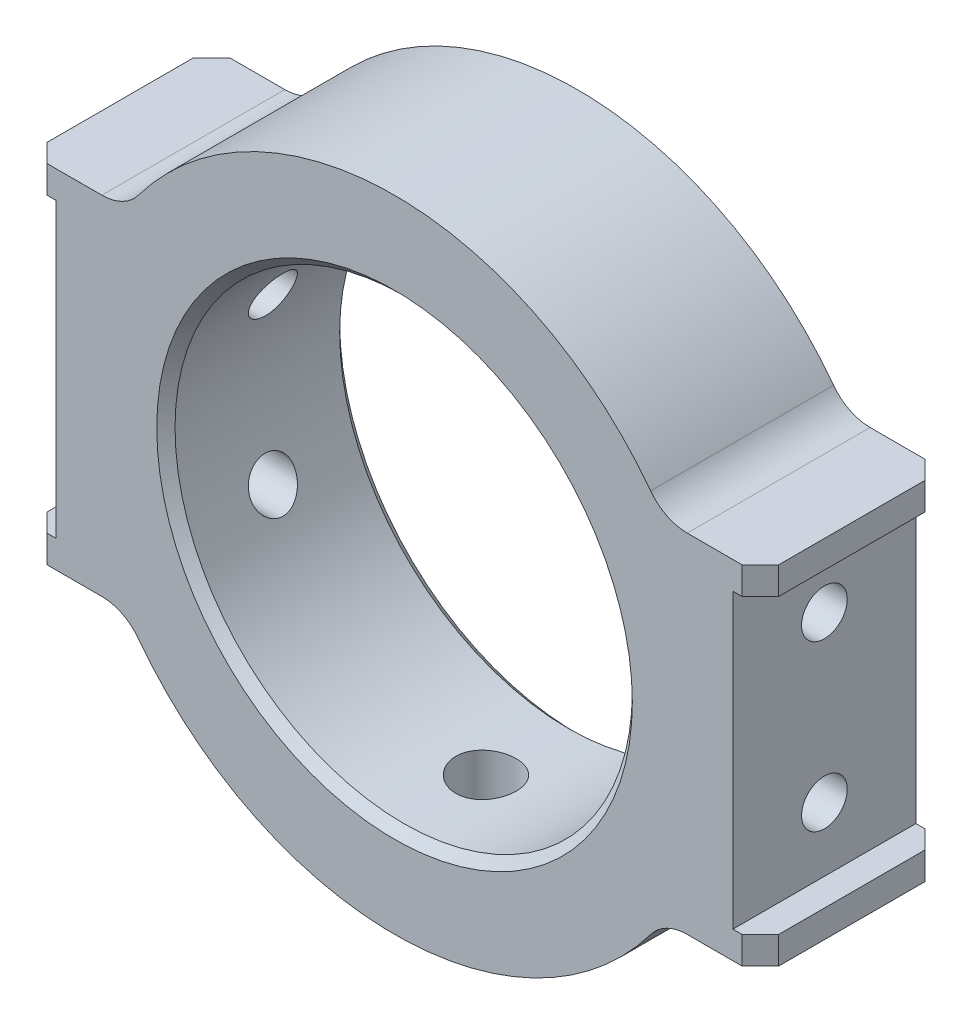
from build123d import *

# Parameters (mm, degrees)
SKETCH1_R                  = 17.5
BOSS_EXTRUDE1_DEPTH        = 10
SKETCH2_W                  = 40
SKETCH2_H                  = 19
BOSS_EXTRUDE2_DEPTH        = 10
CHAMFER1_SIZE              = 1
SKETCH3_R                  = 12.5
CUT_EXTRUDE1_DEPTH         = 29.394541729
SKETCH4_W                  = 3
SKETCH4_H                  = 16
CUT_EXTRUDE2_DEPTH         = 29.394541729
M4_TAPPED_HOLE1_D          = 3.3
M4_TAPPED_HOLE1_DEPTH      = 10.1
M4_TAPPED_HOLE1_TIP        = 0.991420021
FILLET1_R                  = 2.5
M3_TAPPED_HOLE1_AT_2_COUNT = 2
M3_TAPPED_HOLE1_AT_2_PITCH = 9
CHAMFER2_SIZE              = 0.5


with BuildPart() as part:
    # Sketch1 → Boss-Extrude1 (new body)
    with BuildSketch(Plane.XY):
        Circle(SKETCH1_R)
    extrude(amount=BOSS_EXTRUDE1_DEPTH)

    # Sketch2 → Boss-Extrude2 (add)
    with BuildSketch(Plane.XY.offset(10)):
        Rectangle(SKETCH2_W, SKETCH2_H)
    extrude(amount=-BOSS_EXTRUDE2_DEPTH)

    # Chamfer1
    chamfer1_edges = [part.edges().sort_by_distance(p)[0] for p in [
        (20, 0, 10),
        (-20, 0, 10),
        (-20, 0, 0),
        (20, 0, 0),
    ]]
    chamfer(chamfer1_edges, length=CHAMFER1_SIZE)

    # Sketch3 → Cut-Extrude1 (cut, through all)
    with BuildSketch(Plane.XY.offset(10)):
        Circle(SKETCH3_R)
    extrude(amount=-CUT_EXTRUDE1_DEPTH, mode=Mode.SUBTRACT)

    # Sketch4 → Cut-Extrude2 (cut, through all)
    with BuildSketch(Plane.XY.offset(10)):
        with Locations((20, 0)):
            Rectangle(SKETCH4_W, SKETCH4_H)
        with Locations((-20, 0)):
            Rectangle(SKETCH4_W, SKETCH4_H)
    extrude(amount=-CUT_EXTRUDE2_DEPTH, mode=Mode.SUBTRACT)

    # M4 Tapped Hole1
    with Locations(Plane.XZ.offset(20.35278131)):
        with Locations((0, 5)):
            Hole(M4_TAPPED_HOLE1_D / 2, depth=M4_TAPPED_HOLE1_DEPTH)
            with Locations((0, 0, -(M4_TAPPED_HOLE1_DEPTH + M4_TAPPED_HOLE1_TIP / 2))):  # 118° drill point
                Cone(0, M4_TAPPED_HOLE1_D / 2, M4_TAPPED_HOLE1_TIP, mode=Mode.SUBTRACT)

    # Fillet1
    fillet1_edges = [part.edges().sort_by_distance(p)[0] for p in [
        (-14.696938457, -9.5, 5),
        (14.696938457, -9.5, 5),
        (14.696938457, 9.5, 5),
        (-14.696938457, 9.5, 5),
    ]]
    fillet(fillet1_edges, radius=FILLET1_R)

    # Sketch7 → M3 Tapped Hole1 (revolve, cut)
    with BuildSketch(Plane(origin=(18.5, -4.5, 5), x_dir=(0, 0, -1), z_dir=(0, 1, 0))):
        Polygon((0, 0), (0, 8.251075774), (1.25, 7.5), (1.25, 0), align=None)
    m3_tapped_hole1 = revolve(axis=Axis((24.85, -4.5, 5), (-1, 0, 0)), mode=Mode.SUBTRACT)

    # M3 Tapped Hole1 at 2: M3 Tapped Hole1 ×2
    with Locations(*[(0, i * M3_TAPPED_HOLE1_AT_2_PITCH, 0) for i in range(1, M3_TAPPED_HOLE1_AT_2_COUNT)]):
        add(m3_tapped_hole1, mode=Mode.SUBTRACT)

    # Mirror1: M3 Tapped Hole1 across plane
    add(m3_tapped_hole1.mirror(Plane(origin=(0, 0, 0), x_dir=(0, 0, 1), z_dir=(1, 0, 0))), mode=Mode.SUBTRACT)

    # Mirror1 copy 1 sketch → Mirror1 copy 1 (revolve, cut)
    with BuildSketch(Plane(origin=(-18.5, 4.5, 5), x_dir=(0, 0, -1), z_dir=(0, 1, 0))):
        Polygon((0, 0), (0, -8.251075774), (1.25, -7.5), (1.25, 0), align=None)
    revolve(axis=Axis((-24.85, 4.5, 5), (-1, 0, 0)), mode=Mode.SUBTRACT)

    # Chamfer2
    chamfer2_edges = [part.edges().sort_by_distance(p)[0] for p in [
        (-12.5, 0, 0),
        (-12.5, 0, 10),
    ]]
    chamfer(chamfer2_edges, length=CHAMFER2_SIZE)


solid = part.part
